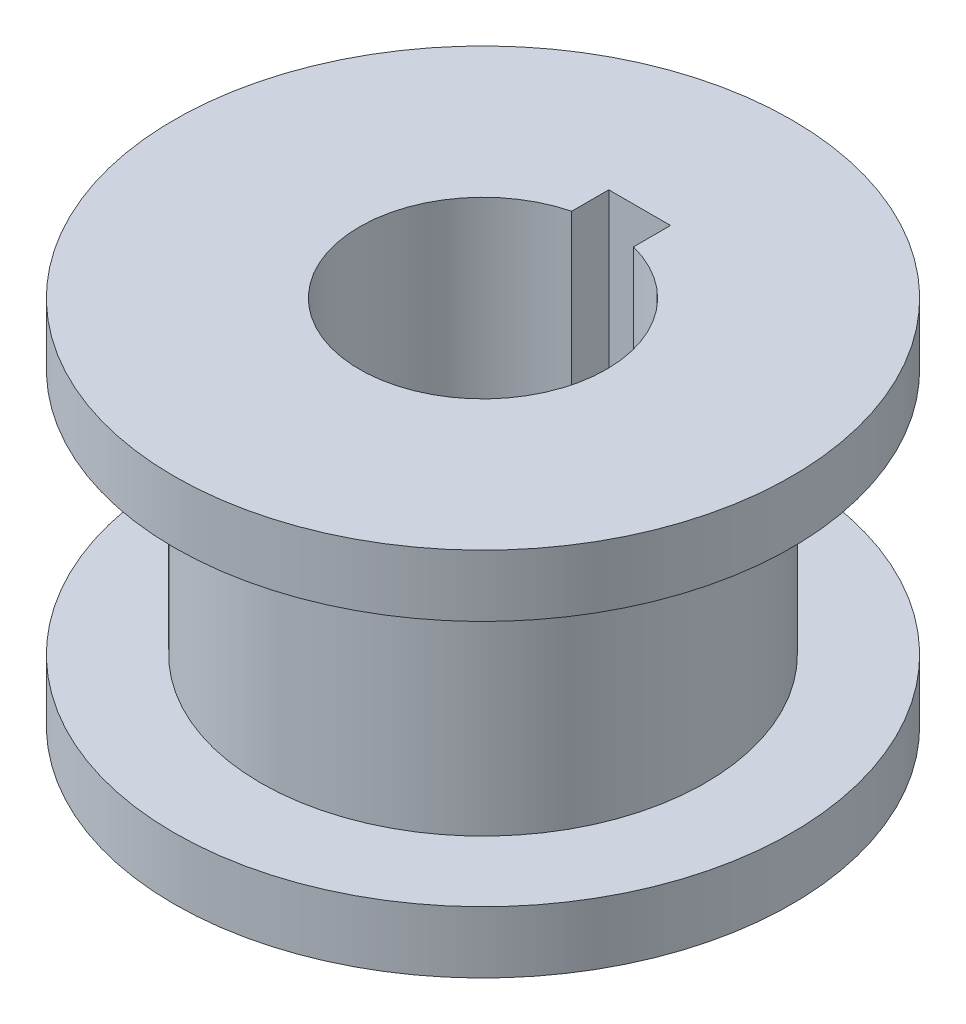
from build123d import *

# Parameters (mm, degrees)
CUT_EXTRUDE1_DEPTH = 47.368092477


with BuildPart() as part:
    # Sketch1 → Revolve1 (revolve)
    with BuildSketch(Plane.XY, mode=Mode.PRIVATE) as revolve1_sk:
        Polygon((-10, 0), (-10, -30), (-25, -30), (-25, -25), (-18, -25), (-18, -5), (-25, -5), (-25, 0), align=None)
    revolve(revolve1_sk.sketch.rotate(Axis((0, 76.758624558, 0), (0, -1, 0)), 270), axis=Axis((0, 76.758624558, 0), (0, -1, 0)))

    # Sketch2 → Cut-Extrude1 (cut, through all)
    with BuildSketch(Plane(origin=(0, 0, 0), x_dir=(1, 0, 0), z_dir=(0, 1, 0))):
        with BuildLine():
            Line((-2.5, 12.682458366), (-2.5, 9.682458366))
            ThreePointArc((-2.5, 9.682458366), (0, 10), (2.5, 9.682458366))
            Line((2.5, 9.682458366), (2.5, 12.682458366))
            Line((2.5, 12.682458366), (-2.5, 12.682458366))
        make_face()
    extrude(amount=-CUT_EXTRUDE1_DEPTH, mode=Mode.SUBTRACT)


solid = part.part
